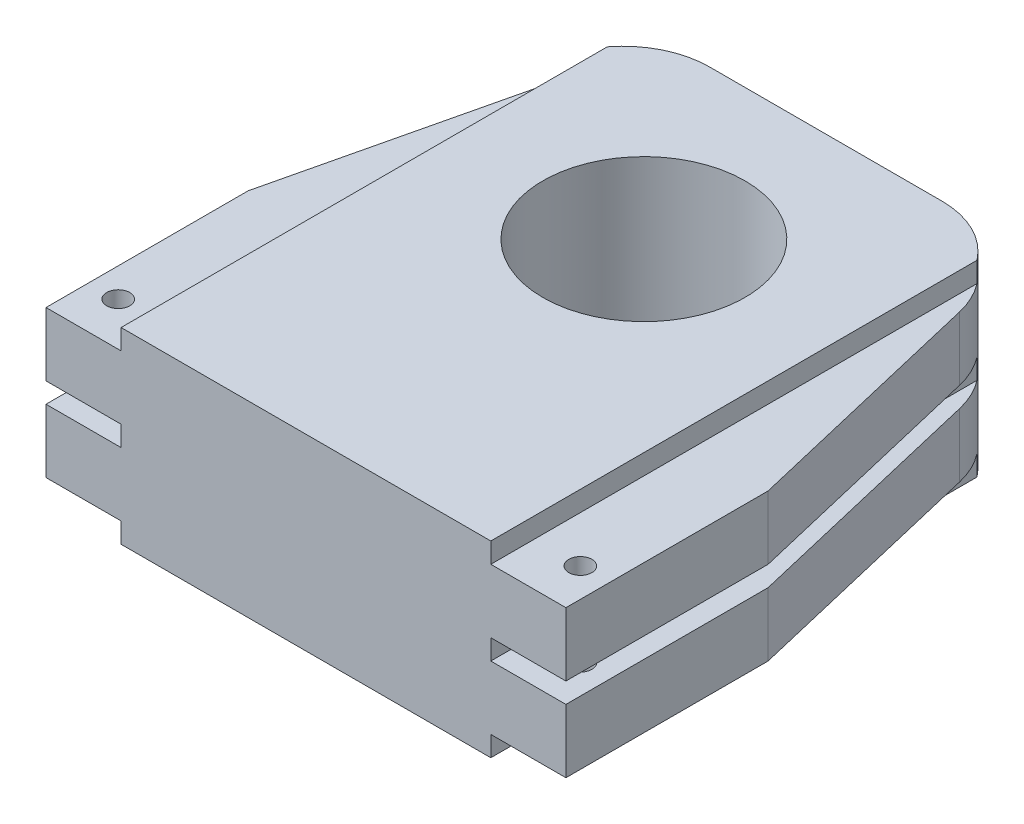
from build123d import *

# Parameters (mm, degrees)
BOSS_EXTRUDE1_DEPTH = 65
SKETCH2_R           = 35
CUT_EXTRUDE1_DEPTH  = 65
SKETCH3_W           = 26
SKETCH3_H           = 7
CUT_EXTRUDE2_DEPTH  = 212.482859826
SKETCH4_R           = 4
CUT_EXTRUDE3_DEPTH  = 210.437341465
SKETCH5_W           = 26
SKETCH5_H           = 7
CUT_EXTRUDE4_DEPTH  = 212.482859826


with BuildPart() as part:
    # Sketch1 → Boss-Extrude1 (new body)
    with BuildSketch(Plane(origin=(0, 0, 0), x_dir=(1, 0, 0), z_dir=(0, 1, 0))):
        with BuildLine():
            Line((-90, 0), (90, 0))
            Line((90, 0), (90, 70))
            Line((90, 70), (69.444464042, 156.905307326))
            ThreePointArc((69.444464042, 156.905307326), (58.862371963, 173.528272565), (40.25, 180))
            Line((40.25, 180), (-40.25, 180))
            ThreePointArc((-40.25, 180), (-58.862371963, 173.528272565), (-69.444464042, 156.905307326))
            Line((-69.444464042, 156.905307326), (-90, 70))
            Line((-90, 70), (-90, 0))
        make_face()
    extrude(amount=BOSS_EXTRUDE1_DEPTH)

    # Sketch2 → Cut-Extrude1 (cut)
    with BuildSketch(Plane(origin=(0, 65, 0), x_dir=(1, 0, 0), z_dir=(0, 1, 0))):
        with Locations(Location((0, 117, 0), (0, 0, 270))):
            Circle(SKETCH2_R)
    extrude(amount=-CUT_EXTRUDE1_DEPTH, mode=Mode.SUBTRACT)

    # Sketch3 → Cut-Extrude2 (cut, through all)
    with BuildSketch(Plane.XY):
        with Locations((77, 3.5)):
            Rectangle(SKETCH3_W, SKETCH3_H)
        with Locations((77, 61.5)):
            Rectangle(SKETCH3_W, SKETCH3_H)
        with Locations((-77, 61.5)):
            Rectangle(SKETCH3_W, SKETCH3_H)
        with Locations((-77, 3.5)):
            Rectangle(SKETCH3_W, SKETCH3_H)
    extrude(amount=-CUT_EXTRUDE2_DEPTH, mode=Mode.SUBTRACT)

    # Sketch4 → Cut-Extrude3 (cut, through all)
    with BuildSketch(Plane.XZ.offset(-7)):
        with Locations((80, -15)):
            Circle(SKETCH4_R)
        with Locations((-80, -15)):
            Circle(SKETCH4_R)
    extrude(amount=-CUT_EXTRUDE3_DEPTH, mode=Mode.SUBTRACT)

    # Sketch5 → Cut-Extrude4 (cut, through all)
    with BuildSketch(Plane.XY):
        with Locations((-77, 32.5)):
            Rectangle(SKETCH5_W, SKETCH5_H)
        with Locations((77, 32.5)):
            Rectangle(SKETCH5_W, SKETCH5_H)
    extrude(amount=-CUT_EXTRUDE4_DEPTH, mode=Mode.SUBTRACT)


solid = part.part
